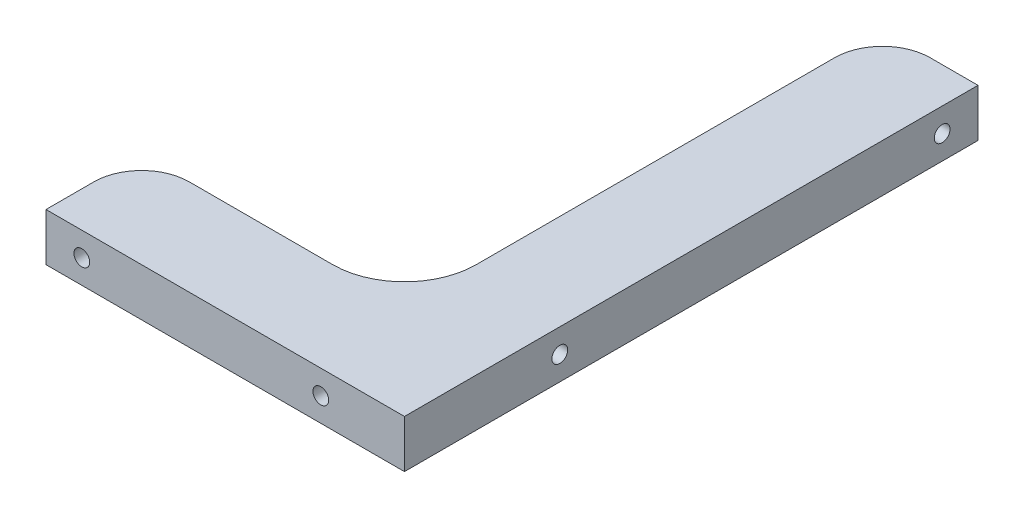
SolidWorks part; units mm, degrees
material "A6061"
ref_plane "前基準面" through (0, 0, 0) normal (0, 0, 1) x (1, 0, 0)
ref_plane "上基準面" through (0, 0, 0) normal (0, 1, 0) x (1, 0, 0)
ref_plane "右基準面" through (0, 0, 0) normal (1, 0, 0) x (0, 0, -1)
sketch "草图1" plane through (0, 0, 0) normal (0, 1, 0) x (1, 0, 0)
  line L1 (-37.5, -60) -> (37.5, -60)
  line L2 (-37.5, -60) -> (-37.5, 60)
  line L3 (-37.5, 60) -> (37.5, 60)
  line L4 (37.5, -60) -> (37.5, 60)
  line L5 (-37.5, -60) -> (37.5, 60) construction
  line L6 (-37.5, 60) -> (37.5, -60) construction
  point P0 (0, 0)
  dimension "D1" = 75
  dimension "D2" = 120
extrude "凸台-拉伸1" add sketch "草图1" along normal mid plane 10
sketch "草图2" plane through (0, 5, 0) normal (0, 1, 0) x (1, 0, 0)
  line L0 (-37.5, 60) -> (-37.5, -60) construction
  line L1 (-37.5, 60) -> (17.5, 60)
  line L2 (-37.5, 60) -> (-37.5, -40)
  line L3 (-37.5, -40) -> (17.5, -40)
  line L4 (17.5, 60) -> (17.5, -40)
  line L5 (37.5, 60) -> (-37.5, 60) construction
  line L6 (37.5, -60) -> (37.5, 60) construction
  line L7 (-37.5, -60) -> (37.5, -60) construction
  dimension "D1" = 20
  dimension "D2" = 20
extrude "切除-拉伸1" cut sketch "草图2" against normal up to surface (10 mm away) up to face at (0, -5, 0)
fillet "圆角1" radius 15 1 edges at (17.5, 0, 40)
fillet "圆角2" radius 10 2 edges at (17.5, 0, -60) (-37.5, 0, 40)
hole_wizard "M4 螺纹孔1" positions "草图3" profile "草图4" tap size "M4" standard "GB"
sketch "草图3" plane through (0, 0, 60) normal (0, 0, 1) x (1, 0, 0)
  line L0 (-37.5, 5) -> (-37.5, -5) construction
  point P0 (-30, 0)
  point P2 (20, 0)
  dimension "D1" = 50
  dimension "D2" = 7.5
sketch "草图4" plane through (-30, 0, 60) normal (1, 0, 0) x (0, -1, 0)
  line L0 (0, 0) -> (0, 11.0914)
  line L1 (0, 11.0914) -> (1.65, 10.1)
  line L2 (1.65, 10.1) -> (1.65, 0)
  line L5 (1.65, 0) -> (0, 0)
  line L10 (0, 11.0914) -> (-1.65, 10.1) construction
  line L11 (0, -6.35) -> (0, 107.95) construction
  dimension "螺纹孔钻头直径" = 3.3
  dimension "螺纹孔钻头深度" = 10.1
  dimension "导头角度" = 118
cosmetic thread "孔螺蚊线1" parameters "D1"=8, "D2"=4
cosmetic thread "孔螺蚊线2" parameters "D1"=8, "D2"=4
hole_wizard "M4 螺纹孔2" positions "草图5" profile "草图6" tap size "M4" standard "GB"
sketch "草图5" plane through (37.5, 0, 0) normal (1, 0, 0) x (0, 0, -1)
  line L0 (60, 5) -> (60, -5) construction
  point P0 (-27.5, 0)
  point P2 (52.5, 0)
  dimension "D1" = 7.5
  dimension "D2" = 80
sketch "草图6" plane through (37.5, 0, 27.5) normal (0, 1, 0) x (0, 0, -1)
  line L0 (0, 0) -> (0, 11.0914)
  line L1 (0, 11.0914) -> (1.65, 10.1)
  line L2 (1.65, 10.1) -> (1.65, 0)
  line L5 (1.65, 0) -> (0, 0)
  line L10 (0, 11.0914) -> (-1.65, 10.1) construction
  line L11 (0, -6.35) -> (0, 107.95) construction
  dimension "螺纹孔钻头直径" = 3.3
  dimension "螺纹孔钻头深度" = 10.1
  dimension "导头角度" = 118
cosmetic thread "孔螺蚊线3" parameters "D1"=8, "D2"=4
cosmetic thread "孔螺蚊线4" parameters "D1"=8, "D2"=4
